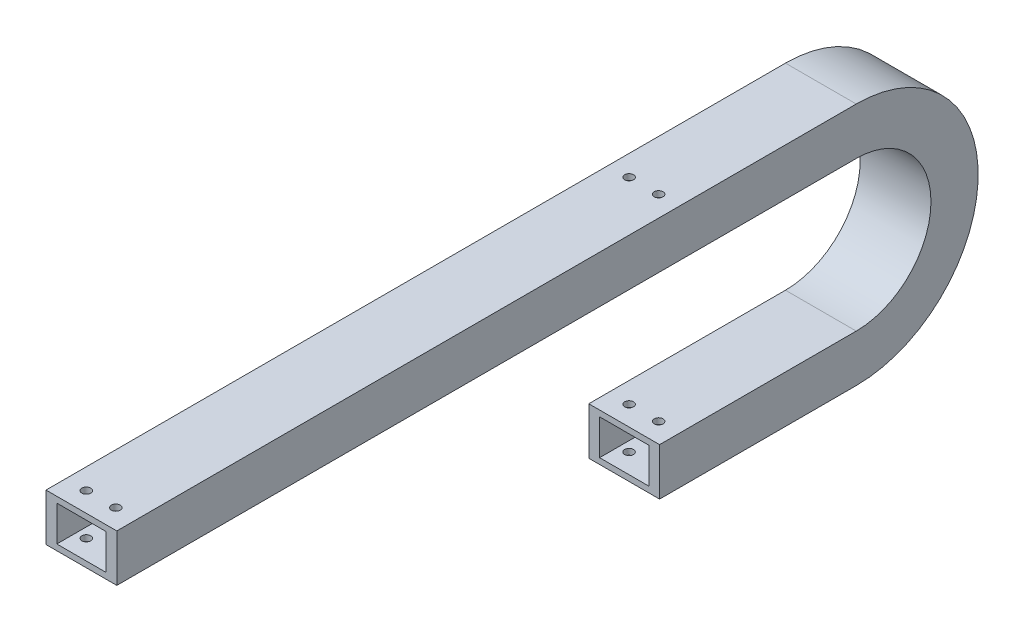
SolidWorks part; units mm, degrees
ref_plane "前视基准面" through (0, 0, 0) normal (0, 0, 1) x (1, 0, 0)
ref_plane "上视基准面" through (0, 0, 0) normal (0, 1, 0) x (1, 0, 0)
ref_plane "右视基准面" through (0, 0, 0) normal (1, 0, 0) x (0, 0, -1)
sketch "草图2" plane through (0, 0, 0) normal (0, 0, 1) x (1, 0, 0)
  line L1 (-18, 12) -> (18, 12)
  line L2 (-18, 12) -> (-18, -12)
  line L3 (-18, -12) -> (18, -12)
  line L4 (18, 12) -> (18, -12)
  line L5 (-18, 12) -> (18, -12) construction
  line L6 (-18, -12) -> (18, 12) construction
  line L7 (-12.5, 9) -> (12.5, 9)
  line L8 (-12.5, 9) -> (-12.5, -9)
  line L9 (-12.5, -9) -> (12.5, -9)
  line L10 (12.5, 9) -> (12.5, -9)
  line L11 (-12.5, 9) -> (12.5, -9) construction
  line L12 (-12.5, -9) -> (12.5, 9) construction
  point P0 (0, 0)
  point P6 (0, 0)
  dimension "D1" = 36
  dimension "D2" = 24
  dimension "D3" = 18
  dimension "D4" = 25
sketch "草图3" plane through (0, 0, 0) normal (1, 0, 0) x (0, 0, -1)
  line L0 (0, 0) -> (100, 0)
  line L1 (-276, 100) -> (100, 100)
  arc A0 (100, 0) -> (100, 100) centre (100, 50) ccw
  dimension "D1" = 50
  dimension "D2" = 100
  dimension "D3" = 376
sweep "扫描1" add profiles "草图2" path "草图3"
sketch "草图4" plane through (0, -12, 0) normal (0, -1, 0) x (1, 0, 0)
  line L0 (18, 276) -> (-18, 276) construction
  line L1 (-18, -100) -> (-18, 276) construction
  line L2 (-18, 0) -> (18, 0) construction
  circle A0 centre (-7.5, -10) radius 2.25
  circle A1 centre (7.5, -10) radius 2.25
  circle A2 centre (-7.5, 266) radius 2.25
  circle A3 centre (7.5, 266) radius 2.25
  dimension "D1" = 15
  dimension "D2" = 10
  dimension "D3" = 10.5
  dimension "D4" = 4.5
  dimension "D5" = 15
  dimension "D6" = 7.5
  dimension "D7" = 10
extrude "切除-拉伸1" cut sketch "草图4" against normal through all
